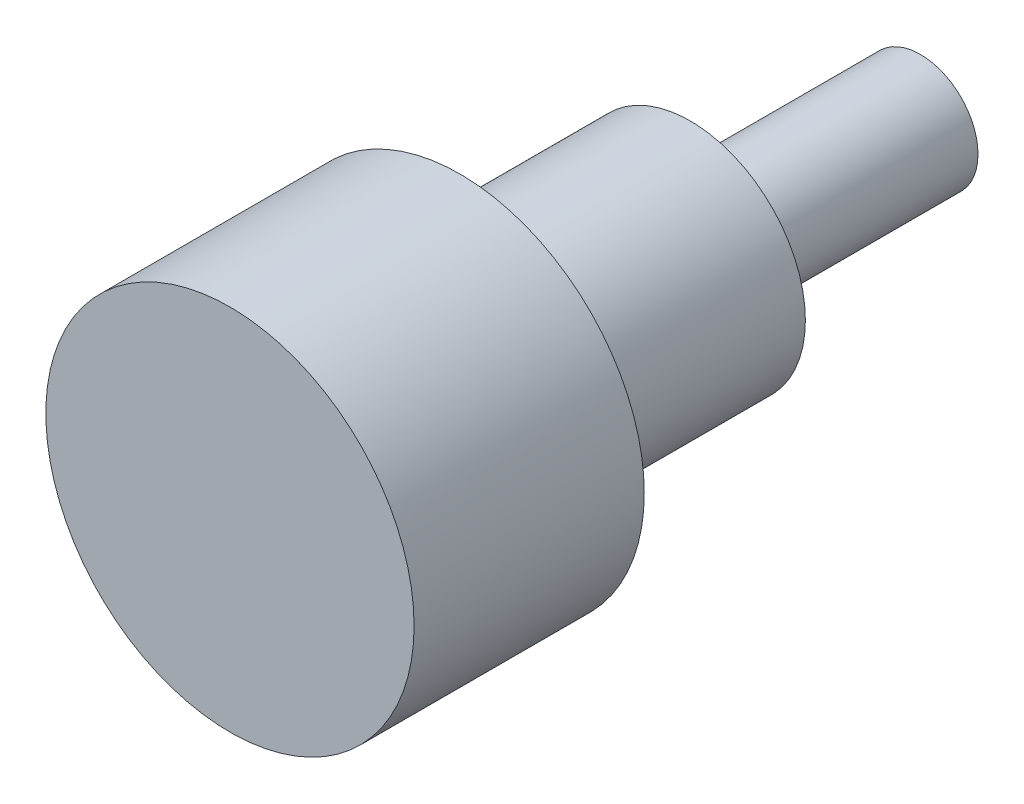
SolidWorks part; units mm, degrees
ref_plane "Front Plane" through (0, 0, 0) normal (0, 0, 1) x (1, 0, 0)
ref_plane "Top Plane" through (0, 0, 0) normal (0, 1, 0) x (1, 0, 0)
ref_plane "Right Plane" through (0, 0, 0) normal (1, 0, 0) x (0, 0, -1)
other "Configuration Table"
sketch "Sketch1" plane through (0, 0, 0) normal (0, 0, 1) x (1, 0, 0)
  circle A0 centre (0, 0) radius 2.5
  dimension "D1" = 5
extrude "Boss-Extrude1" add sketch "Sketch1" along normal blind 10
sketch "Sketch2" plane through (0, 0, 10) normal (0, 0, 1) x (1, 0, 0)
  circle A0 centre (0, 0) radius 5
  dimension "D1" = 10
extrude "Boss-Extrude2" add sketch "Sketch2" along normal blind 10
sketch "Sketch3" plane through (0, 0, 20) normal (0, 0, 1) x (1, 0, 0)
  circle A0 centre (0, 0) radius 8
  dimension "D1" = 16
extrude "Boss-Extrude3" add sketch "Sketch3" along normal blind 10
